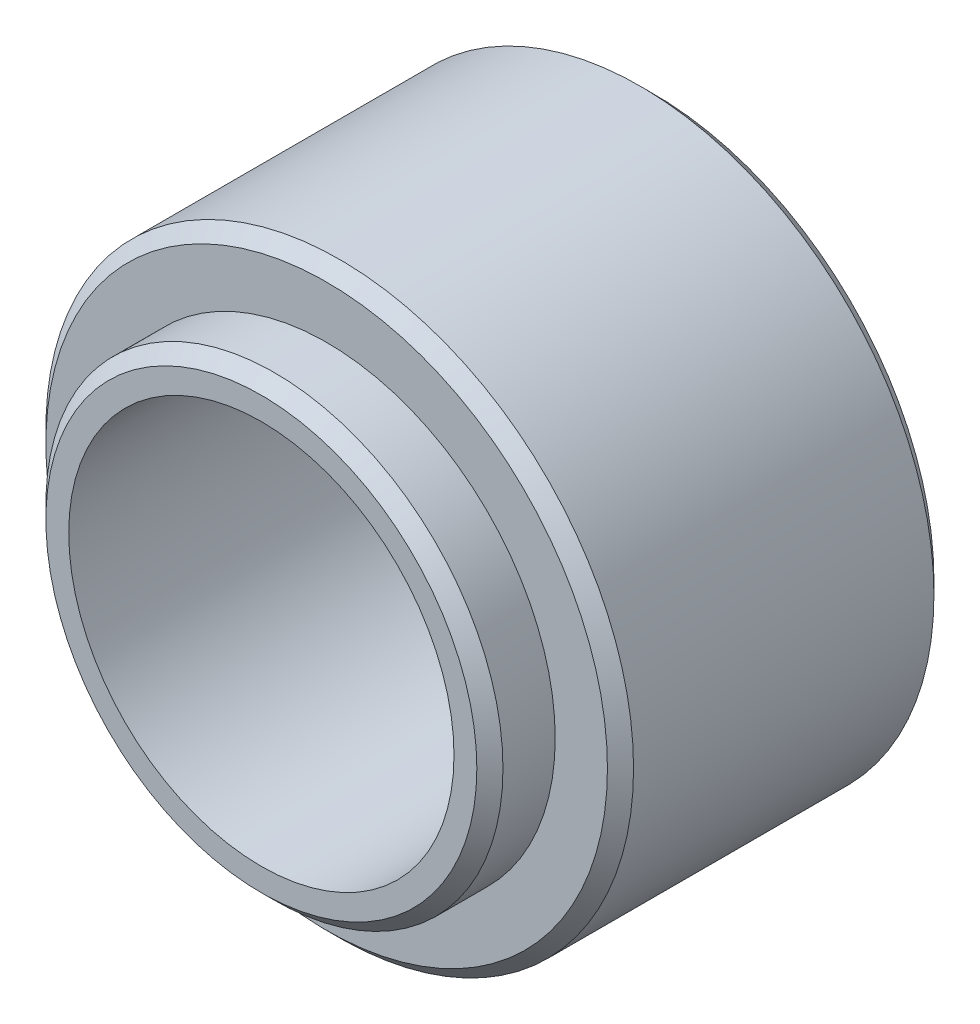
from build123d import *

# Parameters (mm, degrees)
SKETCH1_R           = 22.5
SKETCH1_R_2         = 14.75
BOSS_EXTRUDE1_DEPTH = 25
SKETCH2_R           = 17.5
SKETCH2_R_2         = 14.75
BOSS_EXTRUDE2_DEPTH = 5
CHAMFER2_SIZE       = 1


with BuildPart() as part:
    # Sketch1 → Boss-Extrude1 (new body)
    with BuildSketch(Plane.XY):
        Circle(SKETCH1_R)
        Circle(SKETCH1_R_2, mode=Mode.SUBTRACT)
    extrude(amount=BOSS_EXTRUDE1_DEPTH)

    # Sketch2 → Boss-Extrude2 (add)
    with BuildSketch(Plane.XY.offset(25)):
        Circle(SKETCH2_R)
        Circle(SKETCH2_R_2, mode=Mode.SUBTRACT)
    extrude(amount=BOSS_EXTRUDE2_DEPTH)

    # Chamfer2
    chamfer2_edges = [part.edges().sort_by_distance(p)[0] for p in [
        (-17.5, 0, 30),
        (-22.5, 0, 0),
        (-22.5, 0, 25),
    ]]
    chamfer(chamfer2_edges, length=CHAMFER2_SIZE)


solid = part.part
